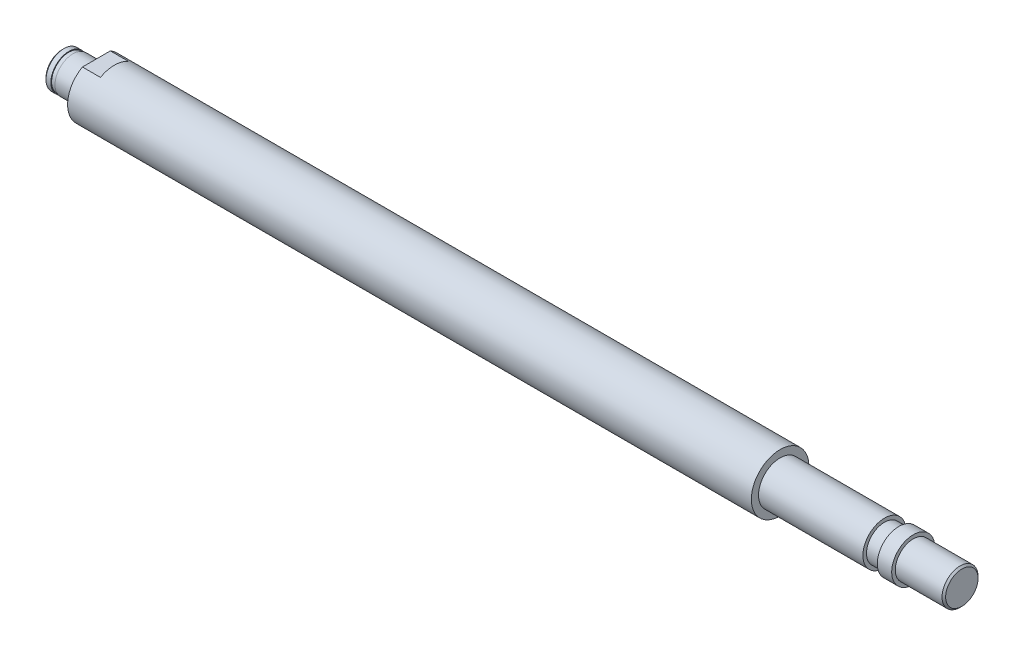
from build123d import *

# Parameters (mm, degrees)
SKETCH2_OUTSIDE_W   = 68.204
SKETCH2_OUTSIDE_H   = 68.204
SKETCH2_OUTSIDE_W_2 = 22.970489672
SKETCH2_OUTSIDE_H_2 = 14
CUT_EXTRUDE1_DEPTH  = 5
CHAMFER1_SIZE       = 0.5


with BuildPart() as part:
    # Sketch1 → Revolve1 (revolve)
    with BuildSketch(Plane.XY, mode=Mode.PRIVATE) as revolve1_sk:
        Polygon((0, 0), (0, 5), (1.85, 5), (1.85, 4.8), (3, 4.8), (3, 5), (9.5, 5), (9.5, 8), (199.5, 8), (199.5, 6), (228.5, 6), (228.5, 5), (232.5, 5), (232.5, 6), (236.5, 6), (236.5, 5), (250, 5), (250, 0), align=None)
    revolve(revolve1_sk.sketch.rotate(Axis((0, 0, 0), (1, 0, 0)), 90), axis=Axis((0, 0, 0), (1, 0, 0)))

    # Sketch2 outside → Cut-Extrude1 (cut)
    with BuildSketch(Plane.ZY.offset(-9.5)):
        Rectangle(SKETCH2_OUTSIDE_W, SKETCH2_OUTSIDE_H)
        Rectangle(SKETCH2_OUTSIDE_W_2, SKETCH2_OUTSIDE_H_2, mode=Mode.SUBTRACT)
    extrude(amount=-CUT_EXTRUDE1_DEPTH, mode=Mode.SUBTRACT)

    # Chamfer1
    chamfer1_edges = [part.edges().sort_by_distance(p)[0] for p in [
        (250, 0, -5),
        (0, 0, -5),
    ]]
    chamfer(chamfer1_edges, length=CHAMFER1_SIZE)


solid = part.part
